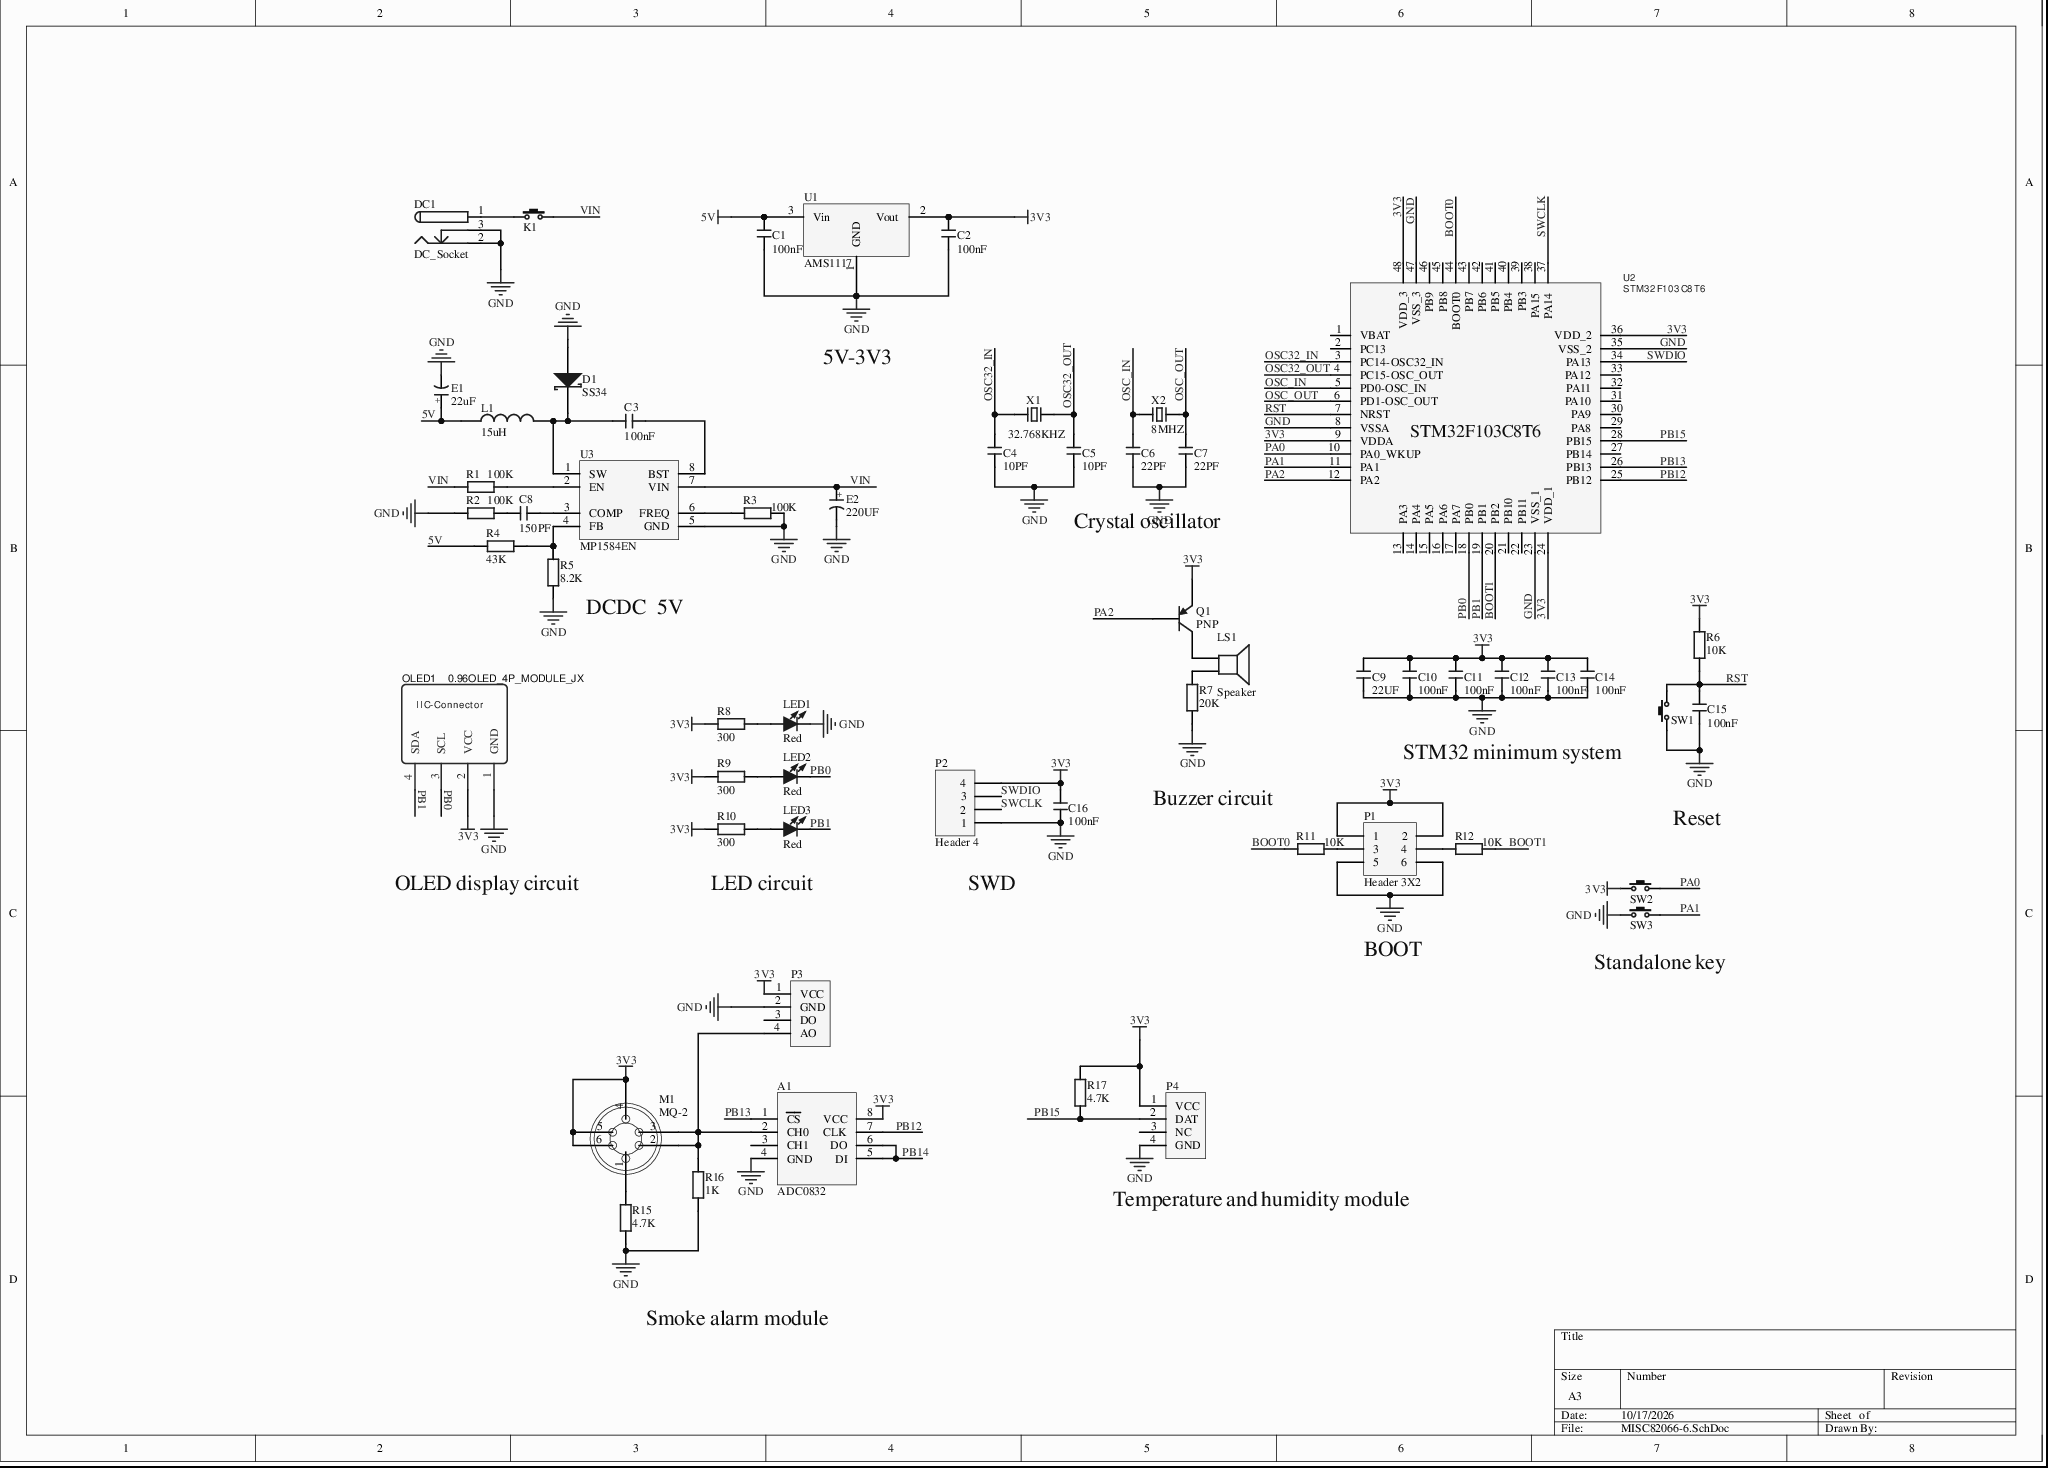
[diagram p0: MISC82066-6.SchDoc]
# Altium project MISC82066-4.PrjPcb
1 sheet, 57 parts. Net scope: global (net labels, ports and power ports of the same name join across sheets).
Board file: MISC82066.PcbDoc

## Sheet MISC82066-6.SchDoc
size A3

### Parts
A1  ADC0832  [DIP8]
C1  100nF  [C 0805_L]
C2  100nF  [C 0805_L]
C3  100nF  [C 0805_L]
C4  10PF  [C 0805_L]
C5  10PF  [C 0805_L]
C6  22PF  [C 0805_L]
C7  22PF  [C 0805_L]
C8  150PF  [C 0805_L]
C9  22UF  [C 0805_L]
C10  100nF  [C 0805_L]
C11  100nF  [C 0805_L]
C12  100nF  [C 0805_L]
C13  100nF  [C 0805_L]
C14  100nF  [C 0805_L]
C15  100nF  [C 0805_L]
C16  100nF  [C 0805_L]
D1  SS34  [SMC]
DC1  DC_Socket  [DC-002]
E1  22uF  [CM A(3*5.4)]
E2  220UF  [CT 5*6 - C]
K1  6x6x5  [TSW DIP-6*6*6_V]  (value not drawn)
L1  15uH  [L 0805]
LED1  Red  [LED 0805G]
LED2  Red  [LED 0805G]
LED3  Red  [LED 0805G]
LS1  Speaker  [PIN2]
M1  MQ-2  [MQ-2]
OLED1  0.96OLED_4P_MODULE_JX  [0.96OLED_4P]
P1  Header 3X2  [HDR2X3]
P2  Header 4  [HDR1X4]
P3  Header 4  [HDR1X4]  (value not drawn)
P4  Header 4  [HDR1X4]  (value not drawn)
Q1  PNP  [SOT-23B_N]
R1  100K  [R 0805_L]
R2  100K  [R 0805_L]
R3  100K  [R 0805_L]
R4  43K  [R 0805_L]
R5  8.2K  [R 0805_L]
R6  10K  [R 0805_L]
R7  20K  [R 0805_L]
R8  300  [R 0805_L]
R9  300  [R 0805_L]
R10  300  [R 0805_L]
R11  10K  [R 0805_L]
R12  10K  [R 0805_L]
R15  4.7K  [R 0805_L]
R16  1K  [R 0805_L]
R17  4.7K  [R 0805_L]
SW1  3x6x5  [TSW SMD-3*6*2.5]  (value not drawn)
SW2  3x6x5  [TSW SMD-3*6*2.5]  (value not drawn)
SW3  3x6x5  [TSW SMD-3*6*2.5]  (value not drawn)
U1  AMS1117  [SOT223]
U2  STM32F103C8T6  [LQFP48 7X7]
U3  MP1584EN  [MP1548EN]
X1  32.768KHZ  [OSC HC-49S]
X2  8MHZ  [OSC HC-49S]

### Nets
3V3: A1.8(VCC) C2.2 C9.2 C10.2 C11.2 C12.2 C13.2 C14.2 C16.2 M1.4(H2) M1.5(A2) M1.6(B2) OLED1.2(VCC) P1.1 P1.2 P2.4 P3.1(VCC) P4.1(VCC) Q1.3(E) R6.1 R8.2 R9.2 R10.2 R17.1 SW2.1 U1.2(Vout) U2.9(VDDA) U2.24(VDD_1) U2.36(VDD_2) U2.48(VDD_3)
5V: C1.2 E1.1(A) L1.1 R4.2 U1.3(Vin)
GND: A1.4(GND) C1.1 C2.1 C4.1 C5.1 C6.1 C7.1 C9.1 C10.1 C11.1 C12.1 C13.1 C14.1 C15.1 C16.1 D1.1(A) DC1.2 DC1.3 E1.2(K) E2.2(K) LED1.2(K) OLED1.1(GND) P1.5 P1.6 P2.1 P3.2(GND) P4.4(GND) R2.1 R3.1 R5.1 R7.2 R15.2 R16.2 SW1.1 SW3.1 U1.1(GND) U2.8(VSSA) U2.23(VSS_1) U2.35(VSS_2) U2.47(VSS_3) U3.5(GND)
BOOT0: R11.2 U2.44(BOOT0)
BOOT1: R12.1 U2.20(PB2)
OSC32_IN: C4.2 U2.3(PC14-OSC32_IN) X1.1
OSC32_OUT: C5.2 U2.4(PC15-OSC_OUT) X1.2
OSC_IN: C6.2 U2.5(PD0-OSC_IN) X2.1
OSC_OUT: C7.2 U2.6(PD1-OSC_OUT) X2.2
PA0: SW2.2 U2.10(PA0_WKUP)
PA1: SW3.2 U2.11(PA1)
PA2: Q1.2(B) U2.12(PA2)
PB0: LED2.2(K) OLED1.3(SCL) U2.18(PB0)
PB1: LED3.2(K) OLED1.4(SDA) U2.19(PB1)
PB12: A1.7(CLK) U2.25(PB12)
PB13: A1.1(~{CS}) U2.26(PB13)
PB14: A1.5(DI) A1.6(DO)
PB15: P4.2(DAT) R17.2 U2.28(PB15)
RST: C15.2 R6.2 SW1.2 U2.7(NRST)
SWCLK: P2.2 U2.37(PA14)
SWDIO: P2.3 U2.34(PA13)
VIN: E2.1(A) K1.2 R1.1 U3.7(VIN)
NetA1_2: A1.2(CH0) M1.2 M1.3(A1) P3.4(AO) R16.1
NetC3_1: C3.1 D1.2(K) L1.2 U3.1(SW)
NetC3_2: C3.2 U3.8(BST)
NetC8_1: C8.1 R2.2
NetC8_2: C8.2 U3.3(COMP)
NetDC1_1: DC1.1 K1.1
NetLED1_1: LED1.1(A) R8.1
NetLED2_1: LED2.1(A) R9.1
NetLED3_1: LED3.1(A) R10.1
NetLS1_1: LS1.1 Q1.1(C)
NetLS1_2: LS1.2 R7.1
NetM1_1: M1.1(H1) R15.1
NetP1_3: P1.3 R11.1
NetP1_4: P1.4 R12.2
NetR1_2: R1.2 U3.2(EN)
NetR3_2: R3.2 U3.6(FREQ)
NetR4_1: R4.1 R5.2 U3.4(FB)

Not connected (* = marked no-connect by the designer): A1 3(CH1); P3 3(DO); P4 3(NC); U2 1(VBAT) 2(PC13) 13(PA3) 14(PA4) 15(PA5) 16(PA6) 17(PA7) 21(PB10) 22(PB11) 27(PB14) 29(PA8) 30(PA9) 31(PA10) 32(PA11) 33(PA12) 38(PA15) 39(PB3) 40(PB4) 41(PB5) 42(PB6) 43(PB7) 45(PB8) 46(PB9)

### Notes on the sheet
- 5V-3V3
- Crystal oscillator
- (near R5) DCDC  5V
- STM32 minimum system
- (near R11) Buzzer circuit
- Reset
- OLED display circuit
- LED circuit
- (near P2) SWD
- BOOT
- (near SW3) Standalone key
- (near P4) Temperature and humidity module
- Smoke alarm module

### Library data of the parts
C1-C16 = C: SMD capacitor; BOM名称: Non-polarized SMD capacitor
D1 = SS34: Schottky diode; 属性: 40V/3A; BOM名称: Schottky diode
E1 = CE_SMD: SMD electrolytic capacitor; BOM名称: SMD electrolytic capacitor
E2 = CS_SMD: SMD solid-state capacitor; BOM名称: SMD solid-state capacitor
K1 = TSW DIP-6x6_V: Side-push through-hole 6x6 tact switch; BOM名称: Through-hole 6x6 tact switch
L1 = L: Low-power SMD inductor; BOM名称: Low-power SMD inductor
LED1-LED3 = LED-SMD: SMD LED; BOM名称: SMD LED
LS1 = Speaker: Loudspeaker; Published: 24-Mar-1999; LatestRevisionDate: 17-Jul-2002; LatestRevisionNote: Re-released for DXP Platform.; PackageReference: PIN2; Publisher: Altium Limited
M1 = MQ-2: Gas sensor
OLED1 = 0.96OLED_4P_MODULE_JX: Manufacturer: null; Contributor: LCSC; Supplier: LCSC; Supplier Part: C9900004566; Manufacturer Part: 0.96OLED_4P_MODULE_JX; JLCPCB Part Class: Extended Part; link: https://so.szlcsc.com/global.html?k=C9900004566&ref=editor; spicePre: O; spiceSymbolName: 0.96OLED_4P_MODULE_JX
P1 = Header 3X2: Header, 3-Pin, Dual row; LatestRevisionDate: 17-Jul-2002; LatestRevisionNote: Re-released for DXP Platform.; Publisher: Altium Limited
P2-P4 = Header 4: Header, 4-Pin; LatestRevisionDate: 17-Jul-2002; LatestRevisionNote: Re-released for DXP Platform.; Publisher: Altium Limited
Q1 = PNP: PNP Bipolar Transistor; Published: 8-Jun-2000; LatestRevisionDate: 29-May-2009; LatestRevisionNote: IPC-7351 Footprint Added.; PackageVersion: Aug-1999; PackageReference: SOT-23B; PackageDescription: 3-Pin SOT-23 Package 0.95 mm Pitch, 2.4 mm Lead Span; Publisher: Altium Limited
R1-R12 R15-R17 = R: SMD resistor; BOM名称: SMD resistor
SW1-SW3 = TSW 3x6: 3x6 tact switch; BOM名称: 3x6 tact switch
U1 = AMS1117: Three-terminal regulator IC
X1 X2 = XTAL-2P: 2-pin passive crystal oscillator; BOM名称: 2-pin passive crystal oscillator